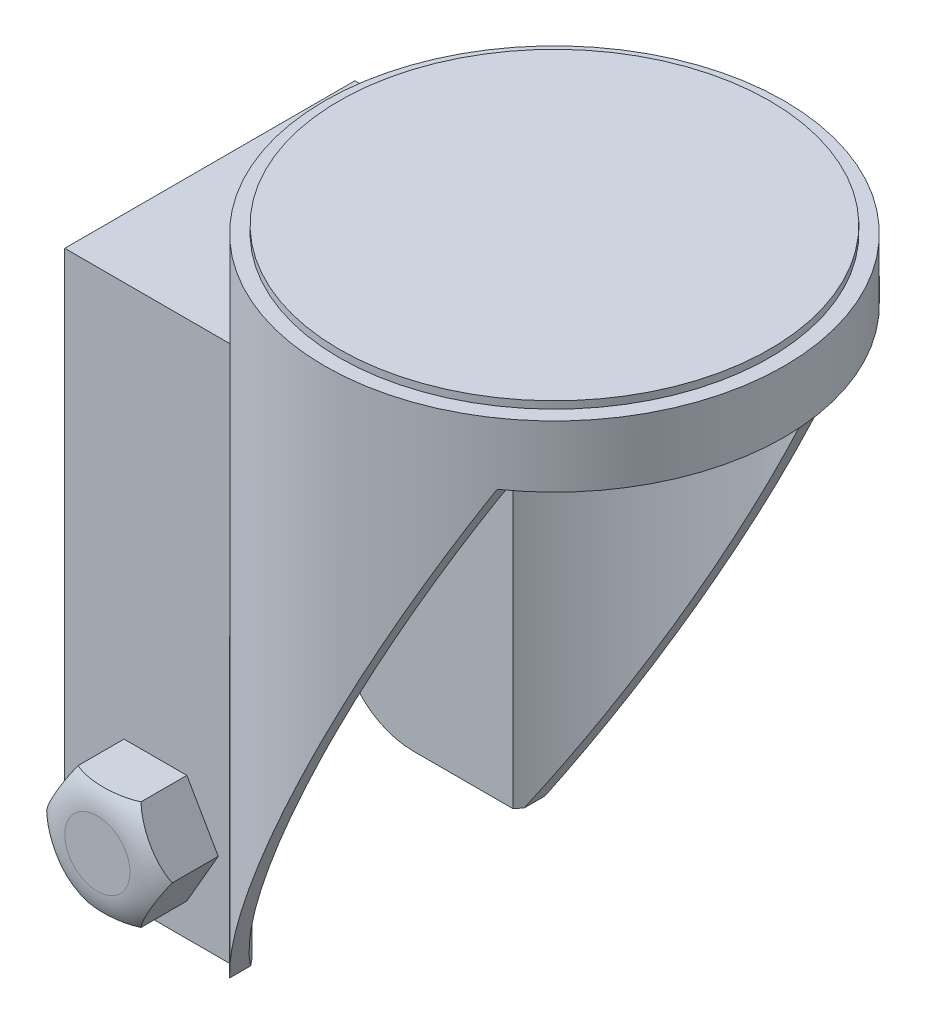
from build123d import *

# Parameters (mm, degrees)
SKETCH2_W               = 36
SKETCH2_H               = 106
CUT_EXTRUDE1_DEPTH      = 95
BOSS_EXTRUDE1_DEPTH     = 47.5
SKETCH4_R               = 29.766666667
CUT_EXTRUDE2_DEPTH      = 144
CUT_EXTRUDE3_DEPTH      = 95
CUT_EXTRUDE3_DEPTH_BACK = 95
SKETCH6_R               = 7
BOSS_EXTRUDE2_DEPTH     = 3
SKETCH8_R               = 9
CUT_EXTRUDE4_DEPTH      = 10


with BuildPart() as part:
    # Sketch1 → Revolve1 (revolve)
    with BuildSketch(Plane(origin=(0, 0, 0), x_dir=(0, 0, -1), z_dir=(1, 0, 0))):
        Polygon((0, -17.975), (-29.666666667, -17.975), (-29.666666667, -109.475), (-31.666666667, -109.475), (-31.666666667, -16.475), (-29.666666667, -16.475), (-29.666666667, -15.475), (0, -15.475), align=None)
    revolve(axis=Axis((0, -15.475, 0), (0, -1, 0)))

    # Sketch2 → Cut-Extrude1 (cut)
    with BuildSketch(Plane(origin=(0, 0, 0), x_dir=(0, 0, -1), z_dir=(1, 0, 0))):
        with Locations((0, -87)):
            Rectangle(SKETCH2_W, SKETCH2_H)
    extrude(amount=-CUT_EXTRUDE1_DEPTH, mode=Mode.SUBTRACT)

    # Sketch3 → Boss-Extrude1 (add)
    with BuildSketch(Plane(origin=(0, 0, 0), x_dir=(0, 0, -1), z_dir=(1, 0, 0))):
        Polygon((-20, -32), (-20, -106), (-18, -106), (-18, -34), (18, -34), (18, -106), (20, -106), (20, -32), align=None)
    extrude(amount=-BOSS_EXTRUDE1_DEPTH)

    # Sketch4 → Cut-Extrude2 (cut)
    with BuildSketch(Plane(origin=(0, -18.475, 0), x_dir=(1, 0, 0), z_dir=(0, 1, 0))):
        with Locations(Location((0, 0, 0), (0, 0, 270))):
            Circle(SKETCH4_R)
    extrude(amount=-CUT_EXTRUDE2_DEPTH, mode=Mode.SUBTRACT)

    # Sketch5 → Cut-Extrude3 (cut, two sides: drawn at the far end of the back side and taken through both)
    with BuildSketch(Plane.XY.offset(-CUT_EXTRUDE3_DEPTH_BACK)):
        with BuildLine():
            Line((-81.666666667, -159.475), (31.666666667, -159.475))
            Line((31.666666667, -159.475), (31.666666667, -24.975))
            Line((31.666666667, -24.975), (18.095238095, -24.975))
            Line((18.095238095, -24.975), (-23.03030303, -106))
            Line((-23.03030303, -106), (-37.5, -106))
            ThreePointArc((-37.5, -106), (-44.571067812, -103.071067812), (-47.5, -96))
            Line((-47.5, -96), (-47.5, -61.653061224))
            Line((-47.5, -61.653061224), (-81.666666667, -106))
            Line((-81.666666667, -106), (-81.666666667, -159.475))
        make_face()
    extrude(amount=CUT_EXTRUDE3_DEPTH + CUT_EXTRUDE3_DEPTH_BACK, mode=Mode.SUBTRACT)

    # Sketch6 → Boss-Extrude2 (add)
    with BuildSketch(Plane.XY.offset(-20)):
        with Locations((-35, -94)):
            Circle(SKETCH6_R)
    extrude(amount=-BOSS_EXTRUDE2_DEPTH)

    # Sketch7 → Revolve2 (revolve)
    with BuildSketch(Plane(origin=(-35, 0, 0), x_dir=(0, 0, -1), z_dir=(1, 0, 0)), mode=Mode.PRIVATE) as revolve2_sk:
        with BuildLine():
            Line((-28, -94), (-28, -89.5))
            ThreePointArc((-28, -89.5), (-27.442646012, -87.053268439), (-26, -85))
            Line((-26, -85), (-20, -85))
            Line((-20, -85), (-20, -94))
            Line((-20, -94), (-28, -94))
        make_face()
    revolve(revolve2_sk.sketch.rotate(Axis((-35, -94, 20), (0, 0, 1)), 90), axis=Axis((-35, -94, 20), (0, 0, 1)))

    # Sketch8 → Cut-Extrude4 (cut)
    with BuildSketch(Plane.XY.offset(20)):
        with Locations((-35, -94)):
            Circle(SKETCH8_R)
        Polygon((-43.660254038, -94), (-39.330127019, -101.5), (-30.669872981, -101.5), (-26.339745962, -94), (-30.669872981, -86.5), (-39.330127019, -86.5), align=None, mode=Mode.SUBTRACT)
    extrude(amount=CUT_EXTRUDE4_DEPTH, mode=Mode.SUBTRACT)


solid = part.part
